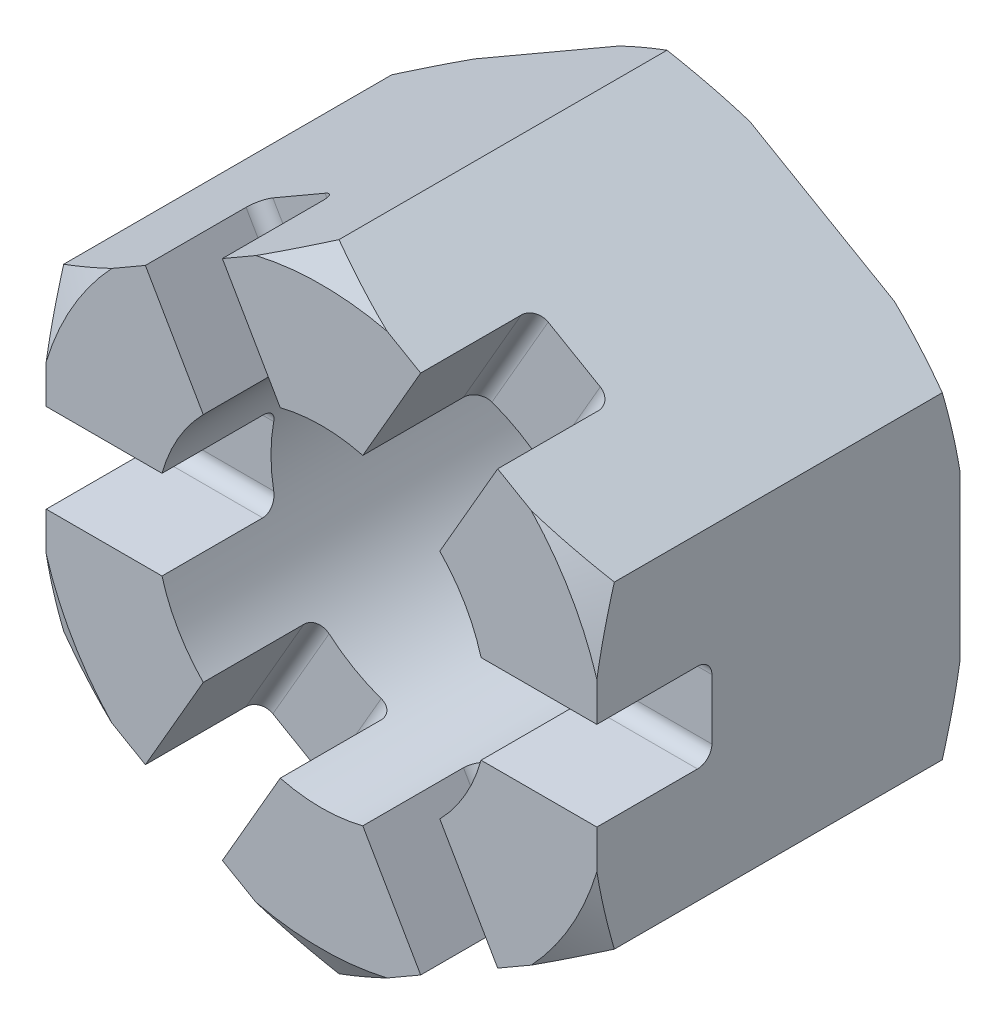
SolidWorks part; units mm, degrees
ref_plane "基准面1" through (0, 0, 0) normal (0, 0, 1) x (1, 0, 0)
ref_plane "基准面2" through (0, 0, 0) normal (0, 1, 0) x (1, 0, 0)
ref_plane "基准面3" through (0, 0, 0) normal (1, 0, 0) x (0, 0, -1)
sketch "尺寸草图" plane through (0, 0, 0) normal (0, 0, 1) x (1, 0, 0)
  line L0 (0, 0) -> (55, 0) construction
  line L1 (60.79, 0) -> (99.69, 0) construction
  line L2 (99.69, 0) -> (150.79, 0) construction
  line L3 (-30.2857, 0) -> (4, 0) construction
  line L4 (0, 0) -> (60.79, 0) construction
  line L5 (-30.2857, 0) -> (-30.2857, 26.5) construction
  point P3 (36, 0)
  point P4 (4, 0)
  point P5 (60.79, 0)
  point P6 (34.7, 0)
  point P8 (55, 0)
  point P15 (84.49, 0)
  point P16 (108.19, 0)
  dimension "D1" = 34.2857
  dimension "D" = 36
  dimension "P" = 4
  dimension "e(min)" = 60.79
  dimension "m(max)" = 34.7
  dimension "s(max)" = 55
  dimension "da(max)" = 38.9
  dimension "dw(min)" = 51.1
  dimension "w(max)" = 23.7
  dimension "n(max)" = 8.5
  dimension "m´(min)" = 26.5
sketch "草图1" plane through (0, 0, 0) normal (0, 0, 1) x (1, 0, 0)
  line L0 (-26.3228, 0) -> (26.3228, 0) construction
  line L1 (0, 30.395) -> (0, -30.395) construction
  line L3 (0, 30.395) -> (-26.3228, 15.1975)
  line L4 (-26.3228, 15.1975) -> (-26.3228, -15.1975)
  line L5 (-26.3228, -15.1975) -> (0, -30.395)
  line L6 (0, -30.395) -> (26.3228, -15.1975)
  line L7 (26.3228, -15.1975) -> (26.3228, 15.1975)
  line L8 (26.3228, 15.1975) -> (0, 30.395)
  circle A0 centre (0, 0) radius 26.3228 construction
  circle A1 centre (0, 0) radius 15.835
  dimension "D" = 31.67
  dimension "e" = 60.79
extrude "基体-拉伸" add sketch "草图1" along normal blind 34.7
cosmetic thread "装饰螺纹线1" parameters "D2"=36
sketch "草图2" plane through (0, 0, 0) normal (0, 0, -1) x (-1, 0, 0)
  circle A0 centre (0, 0) radius 27.5
  circle A1 centre (0, 0) radius 15.835 construction
  dimension "s" = 55
extrude "切除-拉伸1" cut sketch "草图2" against normal through all draft 60 flip side to cut
sketch "草图3" plane through (0, 0, 34.7) normal (0, 0, 1) x (1, 0, 0)
  circle A0 centre (0, 0) radius 27.5
  dimension "D1" = 55
extrude "切除-拉伸2" cut sketch "草图3" against normal through all draft 60 flip side to cut
sketch "草图6" plane through (26.3228, 0, 0) normal (1, 0, 0) x (0, 0, -1)
  line L0 (-14.9451, 0) -> (3.4921, 0) construction
  line L1 (-34.7, 0) -> (0, 0) construction
  line L3 (-34.7, -7.9598) -> (-34.7, 7.9598) construction
  line L4 (-34.7, -4.25) -> (-34.7, 4.25)
  line L5 (-34.7, 4.25) -> (-25.075, 4.25)
  line L6 (-23.7, -2.875) -> (-23.7, 2.875)
  line L7 (0, -7.9598) -> (0, 7.9598) construction
  line L8 (-34.7, -4.25) -> (-25.075, -4.25)
  arc A0 (-25.075, 4.25) -> (-23.7, 2.875) centre (-25.075, 2.875) cw
  arc A1 (-25.075, -4.25) -> (-23.7, -2.875) centre (-25.075, -2.875) ccw
  point P14 (-23.7, 4.25)
  point P17 (-23.7, -4.25)
  dimension "D1" = 1.375
  dimension "W" = 23.7
  dimension "n" = 4.25
extrude "切除-拉伸3" cut sketch "草图6" against normal through all
pattern_circular "阵列(圆周)1" count 3 over 360 about axis through (0, 0, 0) along (0, 0, 1) of "切除-拉伸3"
chamfer "倒角1" distance 0.5768 angle 45 1 edges at (15.835, 0, 0)
